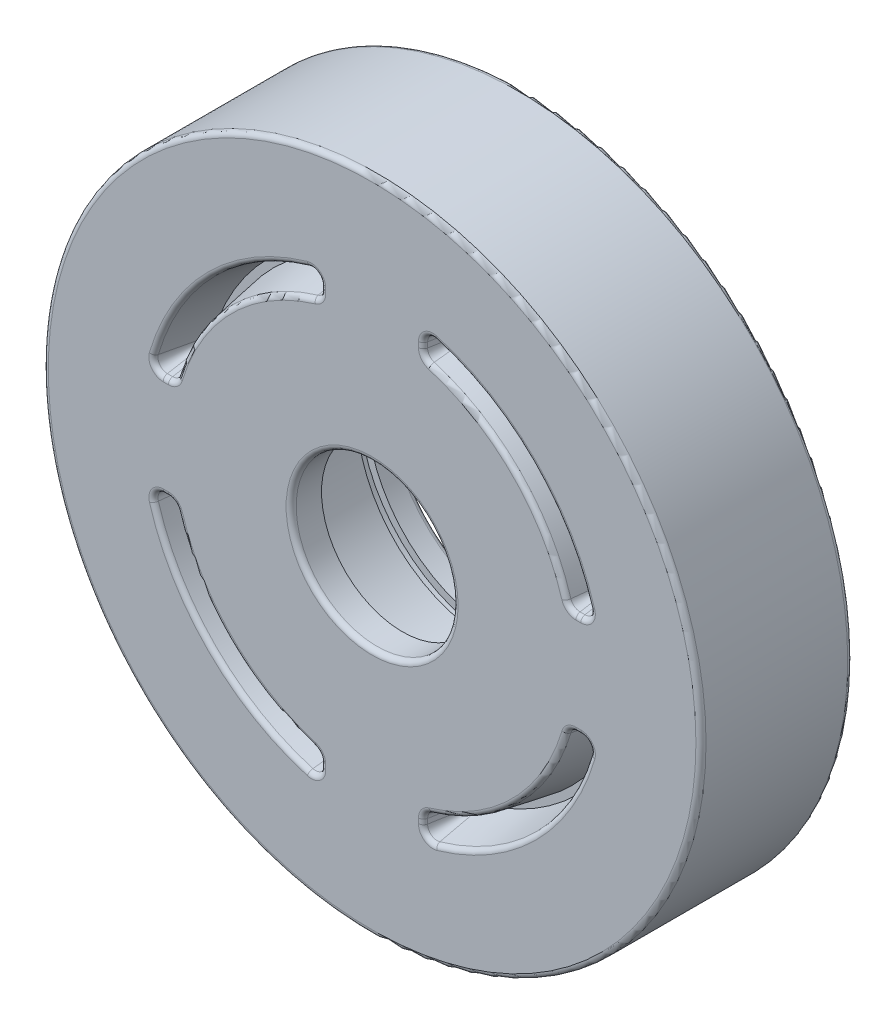
from build123d import *

# Parameters (mm, degrees)
SKETCH1_R                = 65
BOSS_EXTRUDE1_DEPTH      = 15
SKETCH2_R                = 16
CUT_EXTRUDE1_DEPTH       = 6
SKETCH3_R                = 22.5
CUT_EXTRUDE2_DEPTH       = 2
SKETCH4_R                = 26
CUT_EXTRUDE3_DEPTH       = 15
SKETCH5_R                = 27.5
CUT_EXTRUDE4_DEPTH       = 2
SKETCH6_R                = 26
CUT_EXTRUDE5_DEPTH       = 96.262794416
FILLET1_R                = 1
CUT_EXTRUDE6_DEPTH       = 10
CUT_EXTRUDE6_DRAFT       = -10
CIRPATTERN1_COPY_1_DEPTH = 10
CIRPATTERN1_COPY_1_DRAFT = -10
CIRPATTERN1_COPY_2_DEPTH = 10
CIRPATTERN1_COPY_2_DRAFT = -10
CIRPATTERN1_COPY_3_DEPTH = 10
CIRPATTERN1_COPY_3_DRAFT = -10
MIRROR1_COPY_1_DEPTH     = 10
MIRROR1_COPY_1_DRAFT     = -10
MIRROR1_COPY_2_DEPTH     = 10
MIRROR1_COPY_2_DRAFT     = -10
MIRROR1_COPY_3_DEPTH     = 10
MIRROR1_COPY_3_DRAFT     = -10
MIRROR1_COPY_4_DEPTH     = 10
MIRROR1_COPY_4_DRAFT     = -10
FILLET2_R                = 1
SKETCH8_R                = 1.5
CUT_EXTRUDE7_DEPTH       = 10


with BuildPart() as part:
    # Sketch1 → Boss-Extrude1 (new, symmetric)
    with BuildSketch(Plane.XY):
        Circle(SKETCH1_R)
    extrude(amount=BOSS_EXTRUDE1_DEPTH, both=True)

    # Sketch2 → Cut-Extrude1 (cut)
    with BuildSketch(Plane.XY.offset(15)):
        Circle(SKETCH2_R)
    extrude(amount=-CUT_EXTRUDE1_DEPTH, mode=Mode.SUBTRACT)

    # Sketch3 → Cut-Extrude2 (cut)
    with BuildSketch(Plane.XY.offset(9)):
        Circle(SKETCH3_R)
    extrude(amount=-CUT_EXTRUDE2_DEPTH, mode=Mode.SUBTRACT)

    # Sketch4 → Cut-Extrude3 (cut)
    with BuildSketch(Plane.XY.offset(7)):
        Circle(SKETCH4_R)
    extrude(amount=-CUT_EXTRUDE3_DEPTH, mode=Mode.SUBTRACT)

    # Sketch5 → Cut-Extrude4 (cut)
    with BuildSketch(Plane.XY.offset(-8)):
        Circle(SKETCH5_R)
    extrude(amount=-CUT_EXTRUDE4_DEPTH, mode=Mode.SUBTRACT)

    # Sketch6 → Cut-Extrude5 (cut, through all)
    with BuildSketch(Plane.XY.offset(-10)):
        Circle(SKETCH6_R)
    extrude(amount=-CUT_EXTRUDE5_DEPTH, mode=Mode.SUBTRACT)

    # Fillet1
    fillet1_edges = [part.edges().sort_by_distance(p)[0] for p in [
        (-65, 0, -15),
        (-65, 0, 15),
    ]]
    fillet(fillet1_edges, radius=FILLET1_R)


with BuildPart() as cut_extrude6_tool:
    # Sketch7 → Cut-Extrude6 (with draft: the straight prism first)
    with BuildSketch(Plane(origin=(0, 0, -15), x_dir=(-1, 0, 0), z_dir=(0, 0, -1))):
        with BuildLine():
            Line((-10, 40.249223595), (-10, 41.291645644))
            ThreePointArc((-10, 41.291645644), (-10.799225056, 42.891064143), (-12.558139535, 43.212187302))
            ThreePointArc((-12.558139535, 43.212187302), (-31.802817419, 31.836783823), (-43.198757359, 12.604259701))
            ThreePointArc((-43.198757359, 12.604259701), (-42.873365328, 10.81385122), (-41.245763196, 10))
            Line((-41.245763196, 10), (-40.274876119, 10))
            ThreePointArc((-40.274876119, 10), (-39.05957117, 10.402885565), (-38.325609337, 11.451972274))
            ThreePointArc((-38.325609337, 11.451972274), (-28.275635814, 28.292904046), (-11.428571429, 38.3325939))
            ThreePointArc((-11.428571429, 38.3325939), (-10.396432549, 39.053994986), (-10, 40.249223595))
        make_face()
    extrude(amount=-CUT_EXTRUDE6_DEPTH)
    # Cut-Extrude6: the draft: its side faces are tilted about the plane it starts from
    cut_extrude6_sides = [cut_extrude6_tool.faces().sort_by_distance(p)[0] for p in [
        (28.275635814, 28.292904046, -10),
        (10.396432549, 39.053994986, -10),
        (10, 40.77043462, -10),
        (10.799225056, 42.891064143, -10),
        (31.802817419, 31.836783823, -10),
        (42.873365328, 10.81385122, -10),
        (40.760319658, 10, -10),
        (39.05957117, 10.402885565, -10),
    ]]
    draft(cut_extrude6_sides, Plane(origin=(0, 0, -15), x_dir=(-1, 0, 0), z_dir=(0, 0, -1)), CUT_EXTRUDE6_DRAFT)


with BuildPart() as part_1:
    add(part.part)

    # Cut-Extrude6: cut by cut_extrude6_tool
    add(cut_extrude6_tool.part, mode=Mode.SUBTRACT)


with BuildPart() as cirpattern1_copy_1_tool:
    # CirPattern1 copy 1 sketch → CirPattern1 copy 1 (with draft: the straight prism first)
    with BuildSketch(Plane(origin=(0, 0, -15), x_dir=(0, -1, 0), z_dir=(0, 0, -1))):
        with BuildLine():
            Line((-10, 40.249223595), (-10, 41.291645644))
            ThreePointArc((-10, 41.291645644), (-10.799225056, 42.891064143), (-12.558139535, 43.212187302))
            ThreePointArc((-12.558139535, 43.212187302), (-31.802817419, 31.836783823), (-43.198757359, 12.604259701))
            ThreePointArc((-43.198757359, 12.604259701), (-42.873365328, 10.81385122), (-41.245763196, 10))
            Line((-41.245763196, 10), (-40.274876119, 10))
            ThreePointArc((-40.274876119, 10), (-39.05957117, 10.402885565), (-38.325609337, 11.451972274))
            ThreePointArc((-38.325609337, 11.451972274), (-28.275635814, 28.292904046), (-11.428571429, 38.3325939))
            ThreePointArc((-11.428571429, 38.3325939), (-10.396432549, 39.053994986), (-10, 40.249223595))
        make_face()
    extrude(amount=-CIRPATTERN1_COPY_1_DEPTH)
    # CirPattern1 copy 1: the draft: its side faces are tilted about the plane it starts from
    cirpattern1_copy_1_sides = [cirpattern1_copy_1_tool.faces().sort_by_distance(p)[0] for p in [
        (-28.292904046, 28.275635814, -10),
        (-39.053994986, 10.396432549, -10),
        (-40.77043462, 10, -10),
        (-42.891064143, 10.799225056, -10),
        (-31.836783823, 31.802817419, -10),
        (-10.81385122, 42.873365328, -10),
        (-10, 40.760319658, -10),
        (-10.402885565, 39.05957117, -10),
    ]]
    draft(cirpattern1_copy_1_sides, Plane(origin=(0, 0, -15), x_dir=(0, -1, 0), z_dir=(0, 0, -1)), CIRPATTERN1_COPY_1_DRAFT)


with BuildPart() as part_2:
    add(part_1.part)

    # CirPattern1 copy 1: cut by cirpattern1_copy_1_tool
    add(cirpattern1_copy_1_tool.part, mode=Mode.SUBTRACT)


with BuildPart() as cirpattern1_copy_2_tool:
    # CirPattern1 copy 2 sketch → CirPattern1 copy 2 (with draft: the straight prism first)
    with BuildSketch(Plane(origin=(0, 0, -15), x_dir=(1, 0, 0), z_dir=(0, 0, -1))):
        with BuildLine():
            Line((-10, 40.249223595), (-10, 41.291645644))
            ThreePointArc((-10, 41.291645644), (-10.799225056, 42.891064143), (-12.558139535, 43.212187302))
            ThreePointArc((-12.558139535, 43.212187302), (-31.802817419, 31.836783823), (-43.198757359, 12.604259701))
            ThreePointArc((-43.198757359, 12.604259701), (-42.873365328, 10.81385122), (-41.245763196, 10))
            Line((-41.245763196, 10), (-40.274876119, 10))
            ThreePointArc((-40.274876119, 10), (-39.05957117, 10.402885565), (-38.325609337, 11.451972274))
            ThreePointArc((-38.325609337, 11.451972274), (-28.275635814, 28.292904046), (-11.428571429, 38.3325939))
            ThreePointArc((-11.428571429, 38.3325939), (-10.396432549, 39.053994986), (-10, 40.249223595))
        make_face()
    extrude(amount=-CIRPATTERN1_COPY_2_DEPTH)
    # CirPattern1 copy 2: the draft: its side faces are tilted about the plane it starts from
    cirpattern1_copy_2_sides = [cirpattern1_copy_2_tool.faces().sort_by_distance(p)[0] for p in [
        (-28.275635814, -28.292904046, -10),
        (-10.396432549, -39.053994986, -10),
        (-10, -40.77043462, -10),
        (-10.799225056, -42.891064143, -10),
        (-31.802817419, -31.836783823, -10),
        (-42.873365328, -10.81385122, -10),
        (-40.760319658, -10, -10),
        (-39.05957117, -10.402885565, -10),
    ]]
    draft(cirpattern1_copy_2_sides, Plane(origin=(0, 0, -15), x_dir=(1, 0, 0), z_dir=(0, 0, -1)), CIRPATTERN1_COPY_2_DRAFT)


with BuildPart() as part_3:
    add(part_2.part)

    # CirPattern1 copy 2: cut by cirpattern1_copy_2_tool
    add(cirpattern1_copy_2_tool.part, mode=Mode.SUBTRACT)


with BuildPart() as cirpattern1_copy_3_tool:
    # CirPattern1 copy 3 sketch → CirPattern1 copy 3 (with draft: the straight prism first)
    with BuildSketch(Plane.YX.offset(15)):
        with BuildLine():
            Line((-10, 40.249223595), (-10, 41.291645644))
            ThreePointArc((-10, 41.291645644), (-10.799225056, 42.891064143), (-12.558139535, 43.212187302))
            ThreePointArc((-12.558139535, 43.212187302), (-31.802817419, 31.836783823), (-43.198757359, 12.604259701))
            ThreePointArc((-43.198757359, 12.604259701), (-42.873365328, 10.81385122), (-41.245763196, 10))
            Line((-41.245763196, 10), (-40.274876119, 10))
            ThreePointArc((-40.274876119, 10), (-39.05957117, 10.402885565), (-38.325609337, 11.451972274))
            ThreePointArc((-38.325609337, 11.451972274), (-28.275635814, 28.292904046), (-11.428571429, 38.3325939))
            ThreePointArc((-11.428571429, 38.3325939), (-10.396432549, 39.053994986), (-10, 40.249223595))
        make_face()
    extrude(amount=-CIRPATTERN1_COPY_3_DEPTH)
    # CirPattern1 copy 3: the draft: its side faces are tilted about the plane it starts from
    cirpattern1_copy_3_sides = [cirpattern1_copy_3_tool.faces().sort_by_distance(p)[0] for p in [
        (28.292904046, -28.275635814, -10),
        (39.053994986, -10.396432549, -10),
        (40.77043462, -10, -10),
        (42.891064143, -10.799225056, -10),
        (31.836783823, -31.802817419, -10),
        (10.81385122, -42.873365328, -10),
        (10, -40.760319658, -10),
        (10.402885565, -39.05957117, -10),
    ]]
    draft(cirpattern1_copy_3_sides, Plane.YX.offset(15), CIRPATTERN1_COPY_3_DRAFT)


with BuildPart() as part_4:
    add(part_3.part)

    # CirPattern1 copy 3: cut by cirpattern1_copy_3_tool
    add(cirpattern1_copy_3_tool.part, mode=Mode.SUBTRACT)


with BuildPart() as mirror1_copy_1_tool:
    # Mirror1 copy 1 sketch → Mirror1 copy 1 (with draft: the straight prism first)
    with BuildSketch(Plane(origin=(0, 0, 15), x_dir=(-1, 0, 0), z_dir=(0, 0, 1))):
        with BuildLine():
            Line((-10, -40.249223595), (-10, -41.291645644))
            ThreePointArc((-10, -41.291645644), (-10.799225056, -42.891064143), (-12.558139535, -43.212187302))
            ThreePointArc((-12.558139535, -43.212187302), (-31.802817419, -31.836783823), (-43.198757359, -12.604259701))
            ThreePointArc((-43.198757359, -12.604259701), (-42.873365328, -10.81385122), (-41.245763196, -10))
            Line((-41.245763196, -10), (-40.274876119, -10))
            ThreePointArc((-40.274876119, -10), (-39.05957117, -10.402885565), (-38.325609337, -11.451972274))
            ThreePointArc((-38.325609337, -11.451972274), (-28.275635814, -28.292904046), (-11.428571429, -38.3325939))
            ThreePointArc((-11.428571429, -38.3325939), (-10.396432549, -39.053994986), (-10, -40.249223595))
        make_face()
    extrude(amount=-MIRROR1_COPY_1_DEPTH)
    # Mirror1 copy 1: the draft: its side faces are tilted about the plane it starts from
    mirror1_copy_1_sides = [mirror1_copy_1_tool.faces().sort_by_distance(p)[0] for p in [
        (28.275635814, 28.292904046, 10),
        (10.396432549, 39.053994986, 10),
        (10, 40.77043462, 10),
        (10.799225056, 42.891064143, 10),
        (31.802817419, 31.836783823, 10),
        (42.873365328, 10.81385122, 10),
        (40.760319658, 10, 10),
        (39.05957117, 10.402885565, 10),
    ]]
    draft(mirror1_copy_1_sides, Plane(origin=(0, 0, 15), x_dir=(-1, 0, 0), z_dir=(0, 0, 1)), MIRROR1_COPY_1_DRAFT)


with BuildPart() as part_5:
    add(part_4.part)

    # Mirror1 copy 1: cut by mirror1_copy_1_tool
    add(mirror1_copy_1_tool.part, mode=Mode.SUBTRACT)


with BuildPart() as mirror1_copy_2_tool:
    # Mirror1 copy 2 sketch → Mirror1 copy 2 (with draft: the straight prism first)
    with BuildSketch(Plane(origin=(0, 0, 15), x_dir=(0, -1, 0), z_dir=(0, 0, 1))):
        with BuildLine():
            Line((-10, -40.249223595), (-10, -41.291645644))
            ThreePointArc((-10, -41.291645644), (-10.799225056, -42.891064143), (-12.558139535, -43.212187302))
            ThreePointArc((-12.558139535, -43.212187302), (-31.802817419, -31.836783823), (-43.198757359, -12.604259701))
            ThreePointArc((-43.198757359, -12.604259701), (-42.873365328, -10.81385122), (-41.245763196, -10))
            Line((-41.245763196, -10), (-40.274876119, -10))
            ThreePointArc((-40.274876119, -10), (-39.05957117, -10.402885565), (-38.325609337, -11.451972274))
            ThreePointArc((-38.325609337, -11.451972274), (-28.275635814, -28.292904046), (-11.428571429, -38.3325939))
            ThreePointArc((-11.428571429, -38.3325939), (-10.396432549, -39.053994986), (-10, -40.249223595))
        make_face()
    extrude(amount=-MIRROR1_COPY_2_DEPTH)
    # Mirror1 copy 2: the draft: its side faces are tilted about the plane it starts from
    mirror1_copy_2_sides = [mirror1_copy_2_tool.faces().sort_by_distance(p)[0] for p in [
        (-28.292904046, 28.275635814, 10),
        (-39.053994986, 10.396432549, 10),
        (-40.77043462, 10, 10),
        (-42.891064143, 10.799225056, 10),
        (-31.836783823, 31.802817419, 10),
        (-10.81385122, 42.873365328, 10),
        (-10, 40.760319658, 10),
        (-10.402885565, 39.05957117, 10),
    ]]
    draft(mirror1_copy_2_sides, Plane(origin=(0, 0, 15), x_dir=(0, -1, 0), z_dir=(0, 0, 1)), MIRROR1_COPY_2_DRAFT)


with BuildPart() as part_6:
    add(part_5.part)

    # Mirror1 copy 2: cut by mirror1_copy_2_tool
    add(mirror1_copy_2_tool.part, mode=Mode.SUBTRACT)


with BuildPart() as mirror1_copy_3_tool:
    # Mirror1 copy 3 sketch → Mirror1 copy 3 (with draft: the straight prism first)
    with BuildSketch(Plane.XY.offset(15)):
        with BuildLine():
            Line((-10, -40.249223595), (-10, -41.291645644))
            ThreePointArc((-10, -41.291645644), (-10.799225056, -42.891064143), (-12.558139535, -43.212187302))
            ThreePointArc((-12.558139535, -43.212187302), (-31.802817419, -31.836783823), (-43.198757359, -12.604259701))
            ThreePointArc((-43.198757359, -12.604259701), (-42.873365328, -10.81385122), (-41.245763196, -10))
            Line((-41.245763196, -10), (-40.274876119, -10))
            ThreePointArc((-40.274876119, -10), (-39.05957117, -10.402885565), (-38.325609337, -11.451972274))
            ThreePointArc((-38.325609337, -11.451972274), (-28.275635814, -28.292904046), (-11.428571429, -38.3325939))
            ThreePointArc((-11.428571429, -38.3325939), (-10.396432549, -39.053994986), (-10, -40.249223595))
        make_face()
    extrude(amount=-MIRROR1_COPY_3_DEPTH)
    # Mirror1 copy 3: the draft: its side faces are tilted about the plane it starts from
    mirror1_copy_3_sides = [mirror1_copy_3_tool.faces().sort_by_distance(p)[0] for p in [
        (-28.275635814, -28.292904046, 10),
        (-10.396432549, -39.053994986, 10),
        (-10, -40.77043462, 10),
        (-10.799225056, -42.891064143, 10),
        (-31.802817419, -31.836783823, 10),
        (-42.873365328, -10.81385122, 10),
        (-40.760319658, -10, 10),
        (-39.05957117, -10.402885565, 10),
    ]]
    draft(mirror1_copy_3_sides, Plane.XY.offset(15), MIRROR1_COPY_3_DRAFT)


with BuildPart() as part_7:
    add(part_6.part)

    # Mirror1 copy 3: cut by mirror1_copy_3_tool
    add(mirror1_copy_3_tool.part, mode=Mode.SUBTRACT)


with BuildPart() as mirror1_copy_4_tool:
    # Mirror1 copy 4 sketch → Mirror1 copy 4 (with draft: the straight prism first)
    with BuildSketch(Plane(origin=(0, 0, 15), x_dir=(0, 1, 0), z_dir=(0, 0, 1))):
        with BuildLine():
            Line((-10, -40.249223595), (-10, -41.291645644))
            ThreePointArc((-10, -41.291645644), (-10.799225056, -42.891064143), (-12.558139535, -43.212187302))
            ThreePointArc((-12.558139535, -43.212187302), (-31.802817419, -31.836783823), (-43.198757359, -12.604259701))
            ThreePointArc((-43.198757359, -12.604259701), (-42.873365328, -10.81385122), (-41.245763196, -10))
            Line((-41.245763196, -10), (-40.274876119, -10))
            ThreePointArc((-40.274876119, -10), (-39.05957117, -10.402885565), (-38.325609337, -11.451972274))
            ThreePointArc((-38.325609337, -11.451972274), (-28.275635814, -28.292904046), (-11.428571429, -38.3325939))
            ThreePointArc((-11.428571429, -38.3325939), (-10.396432549, -39.053994986), (-10, -40.249223595))
        make_face()
    extrude(amount=-MIRROR1_COPY_4_DEPTH)
    # Mirror1 copy 4: the draft: its side faces are tilted about the plane it starts from
    mirror1_copy_4_sides = [mirror1_copy_4_tool.faces().sort_by_distance(p)[0] for p in [
        (28.292904046, -28.275635814, 10),
        (39.053994986, -10.396432549, 10),
        (40.77043462, -10, 10),
        (42.891064143, -10.799225056, 10),
        (31.836783823, -31.802817419, 10),
        (10.81385122, -42.873365328, 10),
        (10, -40.760319658, 10),
        (10.402885565, -39.05957117, 10),
    ]]
    draft(mirror1_copy_4_sides, Plane(origin=(0, 0, 15), x_dir=(0, 1, 0), z_dir=(0, 0, 1)), MIRROR1_COPY_4_DRAFT)


with BuildPart() as part_8:
    add(part_7.part)

    # Mirror1 copy 4: cut by mirror1_copy_4_tool
    add(mirror1_copy_4_tool.part, mode=Mode.SUBTRACT)

    # Fillet2
    fillet2_edges = [part_8.edges().sort_by_distance(p)[0] for p in [
        (-39.053994986, 10.396432549, -15),
        (-40.77043462, 10, -15),
        (-42.891064143, 10.799225056, -15),
        (-31.836783823, 31.802817419, -15),
        (-10.81385122, 42.873365328, -15),
        (-10, 40.760319658, -15),
        (-10.402885565, 39.05957117, -15),
        (-28.292904046, 28.275635814, -15),
        (10.396432549, 39.053994986, 15),
        (10, 40.77043462, 15),
        (10.799225056, 42.891064143, 15),
        (31.802817419, 31.836783823, 15),
        (42.873365328, 10.81385122, 15),
        (40.760319658, 10, 15),
        (39.05957117, 10.402885565, 15),
        (28.275635814, 28.292904046, 15),
        (39.053994986, -10.396432549, 15),
        (40.77043462, -10, 15),
        (42.891064143, -10.799225056, 15),
        (31.836783823, -31.802817419, 15),
        (10.81385122, -42.873365328, 15),
        (10, -40.760319658, 15),
        (10.402885565, -39.05957117, 15),
        (28.292904046, -28.275635814, 15),
        (-10.396432549, -39.053994986, 15),
        (-10, -40.77043462, 15),
        (-10.799225056, -42.891064143, 15),
        (-31.802817419, -31.836783823, 15),
        (-42.873365328, -10.81385122, 15),
        (-40.760319658, -10, 15),
        (-39.05957117, -10.402885565, 15),
        (-28.275635814, -28.292904046, 15),
        (-39.053994986, 10.396432549, 15),
        (-40.77043462, 10, 15),
        (-42.891064143, 10.799225056, 15),
        (-31.836783823, 31.802817419, 15),
        (-10.81385122, 42.873365328, 15),
        (-10, 40.760319658, 15),
        (-10.402885565, 39.05957117, 15),
        (-28.292904046, 28.275635814, 15),
        (-26, 0, -15),
        (10.396432549, 39.053994986, -15),
        (10, 40.77043462, -15),
        (10.799225056, 42.891064143, -15),
        (31.802817419, 31.836783823, -15),
        (42.873365328, 10.81385122, -15),
        (40.760319658, 10, -15),
        (39.05957117, 10.402885565, -15),
        (28.275635814, 28.292904046, -15),
        (-16, 0, 15),
        (39.053994986, -10.396432549, -15),
        (40.77043462, -10, -15),
        (42.891064143, -10.799225056, -15),
        (31.836783823, -31.802817419, -15),
        (10.81385122, -42.873365328, -15),
        (10, -40.760319658, -15),
        (10.402885565, -39.05957117, -15),
        (28.292904046, -28.275635814, -15),
        (-10.396432549, -39.053994986, -15),
        (-10, -40.77043462, -15),
        (-10.799225056, -42.891064143, -15),
        (-31.802817419, -31.836783823, -15),
        (-42.873365328, -10.81385122, -15),
        (-40.760319658, -10, -15),
        (-39.05957117, -10.402885565, -15),
        (-28.275635814, -28.292904046, -15),
    ]]
    fillet(fillet2_edges, radius=FILLET2_R)

    # Sketch8 → Cut-Extrude7 (cut)
    with BuildSketch(Plane(origin=(0, 0, -15), x_dir=(-1, 0, 0), z_dir=(0, 0, -1))):
        with Locations((0, 32.5)):
            Circle(SKETCH8_R)
        with Locations((28.145825623, -16.25)):
            Circle(SKETCH8_R)
        with Locations((-28.145825623, -16.25)):
            Circle(SKETCH8_R)
    extrude(amount=-CUT_EXTRUDE7_DEPTH, mode=Mode.SUBTRACT)


solid = part_8.part
